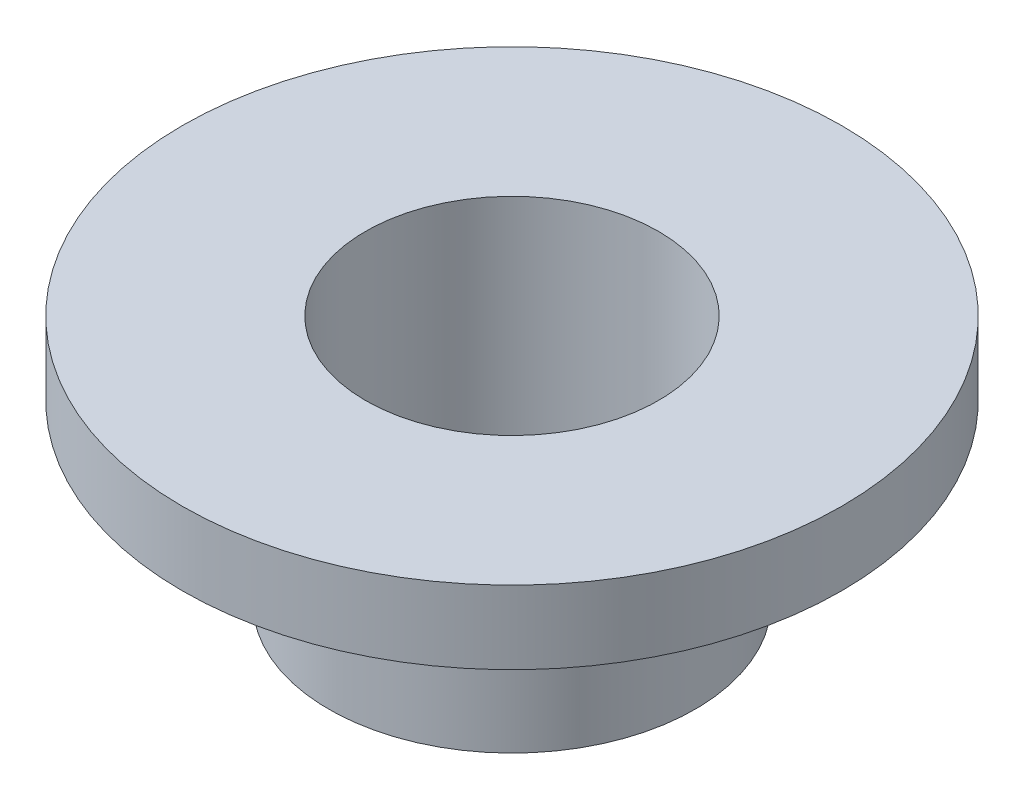
from build123d import *

# Parameters (mm, degrees)
SKETCH_2_R          = 10
CUT_EXTRUDE_1_DEPTH = 26


with BuildPart() as part:
    # 草图1 → 旋转1 (revolve)
    with BuildSketch(Plane.XY, mode=Mode.PRIVATE) as revolve_1_sk:
        Polygon((0, 0), (22.5, 0), (22.5, -5), (12.5, -5), (12.5, -17), (0, -17), align=None)
    revolve(revolve_1_sk.sketch.rotate(Axis((0, 0, 0), (0, 1, 0)), 90), axis=Axis((0, 0, 0), (0, 1, 0)))

    # 草图2 → 切除-拉伸1 (cut)
    with BuildSketch(Plane.XZ.offset(17)):
        with Locations(Location((0, 0, 0), (0, 0, 270))):
            Circle(SKETCH_2_R)
    extrude(amount=-CUT_EXTRUDE_1_DEPTH, mode=Mode.SUBTRACT)


solid = part.part
